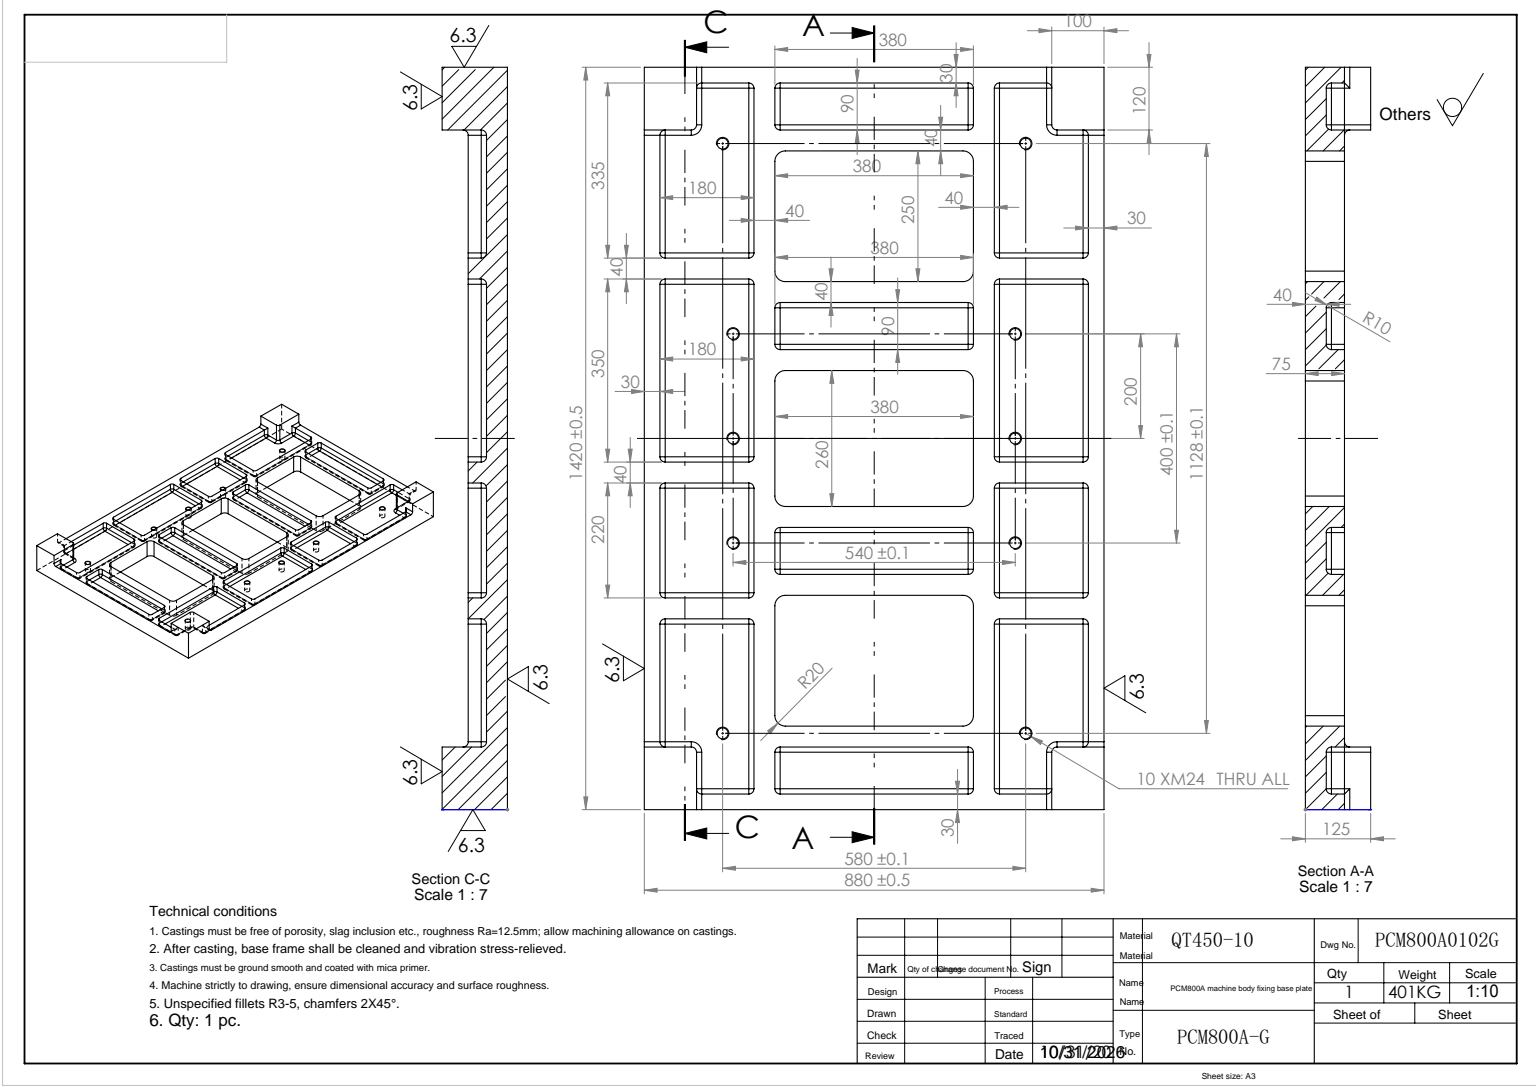
SolidWorks part; units mm, degrees
ref_plane "前视基准面" through (0, 0, 0) normal (0, 0, 1) x (1, 0, 0)
ref_plane "上视基准面" through (0, 0, 0) normal (0, 1, 0) x (1, 0, 0)
ref_plane "右视基准面" through (0, 0, 0) normal (1, 0, 0) x (0, 0, -1)
sketch "草图1" plane through (0, 0, 0) normal (0, 0, 1) x (1, 0, 0)
  line L1 (0, 0) -> (880, 0)
  line L2 (0, 0) -> (0, 75)
  line L3 (0, 75) -> (880, 75)
  line L4 (880, 0) -> (880, 75)
  dimension "D1" = 75
  dimension "D2" = 880
extrude "拉伸1" add sketch "草图1" along normal blind 1420
sketch "草图3" plane through (0, 0, 0) normal (0, -1, 0) x (1, 0, 0)
  line L0 (250, 840) -> (630, 840)
  line L1 (0, 0) -> (880, 0) construction
  line L2 (250, 1260) -> (630, 1260)
  line L3 (250, 1260) -> (250, 1010)
  line L4 (250, 1010) -> (630, 1010)
  line L5 (630, 1260) -> (630, 1010)
  line L6 (250, 410) -> (630, 410)
  line L7 (250, 410) -> (250, 160)
  line L8 (250, 160) -> (630, 160)
  line L9 (630, 410) -> (630, 160)
  line L10 (0, 1420) -> (0, 0) construction
  line L11 (0, 1420) -> (880, 1420) construction
  line L12 (250, 580) -> (630, 580)
  line L15 (250, 580) -> (250, 840)
  line L21 (630, 580) -> (630, 840)
  line L28 (440, 1448.4036) -> (440, -34.642) construction
  dimension "D4" = 160
  dimension "D6" = 250
  dimension "D7" = 250
  dimension "D9" = 380
  dimension "D11" = 190
  dimension "D26" = 380
  dimension "D27" = 190
  dimension "D28" = 380
  dimension "D30" = 190
  dimension "D31" = 170
  dimension "D32" = 170
  dimension "D33" = 440
  dimension "D34" = 160
extrude "切除-拉伸1" cut sketch "草图3" against normal through all
sketch "草图4" plane through (0, 75, 0) normal (0, -1, 0) x (1, 0, 0)
  line L0 (0, 1420) -> (880, 1420) construction
  line L1 (850, 1390) -> (670, 1390)
  line L2 (850, 1390) -> (850, 1055)
  line L3 (850, 1055) -> (670, 1055)
  line L4 (670, 1390) -> (670, 1055)
  line L5 (880, 1420) -> (880, 0) construction
  line L6 (30, 1015) -> (210, 1015)
  line L7 (670, 1015) -> (670, 665)
  line L8 (850, 665) -> (670, 665)
  line L9 (850, 1015) -> (850, 665)
  line L10 (850, 1015) -> (670, 1015)
  line L11 (670, 625) -> (670, 405)
  line L12 (850, 405) -> (670, 405)
  line L13 (850, 625) -> (850, 405)
  line L14 (850, 625) -> (670, 625)
  line L15 (670, 365) -> (670, 30)
  line L16 (850, 30) -> (670, 30)
  line L17 (850, 365) -> (850, 30)
  line L18 (850, 365) -> (670, 365)
  line L19 (30, 1015) -> (30, 665)
  line L20 (440, 1420) -> (440, 0) construction
  line L21 (0, 0) -> (880, 0) construction
  line L22 (210, 1015) -> (210, 665)
  line L23 (210, 1390) -> (210, 1055)
  line L24 (30, 1055) -> (210, 1055)
  line L25 (30, 1390) -> (30, 1055)
  line L26 (30, 1390) -> (210, 1390)
  line L27 (30, 405) -> (210, 405)
  line L28 (30, 365) -> (210, 365)
  line L29 (30, 365) -> (30, 30)
  line L30 (30, 30) -> (210, 30)
  line L31 (210, 365) -> (210, 30)
  line L32 (30, 625) -> (30, 405)
  line L33 (210, 625) -> (210, 405)
  line L34 (30, 665) -> (210, 665)
  line L35 (30, 625) -> (210, 625)
  line L36 (250, 1010) -> (630, 1010) construction
  line L37 (250, 540) -> (630, 540)
  line L38 (250, 970) -> (630, 970)
  line L39 (250, 970) -> (250, 880)
  line L40 (250, 880) -> (630, 880)
  line L41 (630, 970) -> (630, 880)
  line L42 (250, 540) -> (250, 450)
  line L43 (250, 450) -> (630, 450)
  line L44 (630, 540) -> (630, 450)
  line L45 (250, 580) -> (630, 580) construction
  line L46 (250, 160) -> (630, 160) construction
  line L47 (250, 1390) -> (630, 1390)
  line L48 (250, 1390) -> (250, 1300)
  line L49 (250, 1300) -> (630, 1300)
  line L50 (630, 1390) -> (630, 1300)
  line L51 (250, 120) -> (630, 120)
  line L52 (250, 120) -> (250, 30)
  line L53 (250, 30) -> (630, 30)
  line L54 (630, 120) -> (630, 30)
  line L57 (880, 0) -> (0, 0) construction
  dimension "D1" = 180
  dimension "D2" = 30
  dimension "D3" = 30
  dimension "D4" = 335
  dimension "D5" = 350
  dimension "D6" = 40
  dimension "D7" = 40
  dimension "D8" = 40
  dimension "D9" = 335
  dimension "D10" = 220
  dimension "D11" = 180
  dimension "D12" = 180
  dimension "D13" = 40
  dimension "D14" = 40
  dimension "D15" = 90
  dimension "D16" = 380
  dimension "D17" = 40
  dimension "D18" = 90
  dimension "D19" = 380
  dimension "D20" = 40
  dimension "D21" = 180
  dimension "D22" = 30
  dimension "D23" = 30
  dimension "D24" = 30
  dimension "D25" = 90
  dimension "D26" = 40
  dimension "D27" = 380
  dimension "D28" = 40
  dimension "D29" = 90
  dimension "D30" = 40
  dimension "D31" = 380
  dimension "D32" = 30
  dimension "D33" = 30
extrude "切除-拉伸2" cut sketch "草图4" along normal blind 35
fillet "圆角11" radius 20 12 edges at (250, 37.5, 1260) (250, 37.5, 1010) (630, 37.5, 1010) (250, 37.5, 840) (630, 37.5, 840) (630, 37.5, 580) (250, 37.5, 580) (630, 37.5, 410) (630, 37.5, 160) (250, 37.5, 410) (250, 37.5, 160) (630, 37.5, 1260)
fillet "圆角1" radius 10 59 edges at (670, 57.5, 30) (120, 40, 1390) (850, 40, 515) (210, 40, 197.5) (210, 57.5, 30) (670, 57.5, 1055) (670, 57.5, 1390) (250, 40, 925) (250, 57.5, 970) (760, 40, 1015) (670, 57.5, 665) (670, 40, 840) (760, 40, 625) (850, 57.5, 625) (250, 57.5, 540) (440, 40, 540) (670, 57.5, 365) (760, 40, 365) (210, 57.5, 365) (30, 57.5, 30) (30, 40, 197.5) (30, 57.5, 625) (30, 57.5, 1055) (30, 57.5, 1390) (630, 40, 75) (630, 57.5, 30) (850, 57.5, 365) (210, 57.5, 625) (210, 57.5, 405) (210, 57.5, 665) (210, 57.5, 1390) (210, 40, 1222.5) (210, 57.5, 1055) (630, 57.5, 540) (630, 40, 495) (630, 57.5, 450) (630, 57.5, 1390) (630, 40, 1345) (630, 57.5, 970) (630, 40, 925) (850, 57.5, 1015) (850, 40, 840) (850, 57.5, 665) (850, 57.5, 1390) (850, 57.5, 1055) (120, 40, 30) (670, 40, 515) (760, 40, 405) (760, 40, 30) (440, 40, 30) (440, 40, 120) (250, 40, 75) (440, 40, 450) (250, 40, 495) (120, 40, 1055) (120, 40, 665) (440, 40, 880) (760, 40, 1055) (250, 57.5, 30)
hole_wizard "M24 螺纹孔1" positions "3D草图1" profile "草图6" tap size "M24" standard "GB" end condition through all
sketch3d "3D草图1"
  point P0 (150, 40, 146)
  dimension "D1" = 150
  dimension "D2" = 146
sketch "草图6" plane through (150, 40, 146) normal (1, 0, 0) x (0, 0, 1)
  line L0 (0, 0) -> (0, 40)
  line L1 (0, 40) -> (10.5, 40)
  line L2 (10.5, 40) -> (10.5, 0)
  line L5 (10.5, 0) -> (0, 0)
  line L11 (0, -6.35) -> (0, 107.95) construction
  dimension "通孔螺纹孔钻头直径" = 21
  dimension "通孔螺纹孔钻头深度" = 40
cosmetic thread "孔螺蚊线1" parameters "D2"=24
pattern_linear "阵列(线性)2" count 2 spacing 580 along (1, 0, 0) count 2 spacing 1128 along (0, 0, 1) of "M24 螺纹孔1"
hole_wizard "M24 螺纹孔2" positions "3D草图2" profile "草图8" tap size "M24" standard "GB" end condition through all
sketch3d "3D草图2"
  point P0 (170, 40, 510)
  dimension "D1" = 170
  dimension "D2" = 510
sketch "草图8" plane through (170, 40, 510) normal (1, 0, 0) x (0, 0, 1)
  line L0 (0, 0) -> (0, 40)
  line L1 (0, 40) -> (10.5, 40)
  line L2 (10.5, 40) -> (10.5, 0)
  line L5 (10.5, 0) -> (0, 0)
  line L11 (0, -6.35) -> (0, 107.95) construction
  dimension "通孔螺纹孔钻头直径" = 21
  dimension "通孔螺纹孔钻头深度" = 40
cosmetic thread "孔螺蚊线2" parameters "D2"=24
pattern_linear "阵列(线性)3" count 2 spacing 540 along (1, 0, 0) count 3 spacing 200 along (0, 0, 1) of "M24 螺纹孔2"
sketch "草图9" plane through (0, 40, 0) normal (0, 1, 0) x (1, 0, 0)
  line L0 (440, 0) -> (440, -875.7131) construction
  line L1 (0, 0) -> (100, 0)
  line L2 (0, 0) -> (0, -120)
  line L3 (0, -120) -> (100, -120)
  line L4 (100, 0) -> (100, -120)
  line L5 (880, 0) -> (0, 0) construction
  line L6 (0, -710) -> (1254.435, -710) construction
  line L7 (0, -1420) -> (0, 0) construction
  line L8 (780, 0) -> (780, -120)
  line L9 (880, -120) -> (780, -120)
  line L10 (880, 0) -> (880, -120)
  line L11 (880, 0) -> (780, 0)
  line L12 (880, -1420) -> (780, -1420)
  line L13 (880, -1420) -> (880, -1300)
  line L14 (880, -1300) -> (780, -1300)
  line L15 (780, -1420) -> (780, -1300)
  line L16 (100, -1420) -> (100, -1300)
  line L17 (0, -1300) -> (100, -1300)
  line L18 (0, -1420) -> (0, -1300)
  line L19 (0, -1420) -> (100, -1420)
  dimension "D1" = 120
  dimension "D2" = 100
extrude "凸台-拉伸1" add sketch "草图9" along normal blind 85
fillet "圆角12" radius 10 36 edges at (780, 62.5, 30) (780, 42.9289, 32.9289) (850, 62.5, 120) (847.0711, 42.9289, 120) (30, 62.5, 120) (32.9289, 42.9289, 120) (100, 62.5, 30) (100, 42.9289, 32.9289) (30, 62.5, 1300) (32.9289, 42.9289, 1300) (100, 62.5, 1390) (100, 42.9289, 1387.0711) (850, 62.5, 1300) (847.0711, 42.9289, 1300) (780, 62.5, 1390) (780, 42.9289, 1387.0711) (780, 82.5, 120) (865, 75, 120) (780, 75, 15) (780, 40, 80) (810, 40, 120) (100, 82.5, 120) (15, 75, 120) (70, 40, 120) (100, 75, 15) (100, 40, 80) (100, 82.5, 1300) (15, 75, 1300) (70, 40, 1300) (100, 75, 1405) (100, 40, 1340) (780, 82.5, 1300) (865, 75, 1300) (810, 40, 1300) (780, 75, 1405) (780, 40, 1340)
